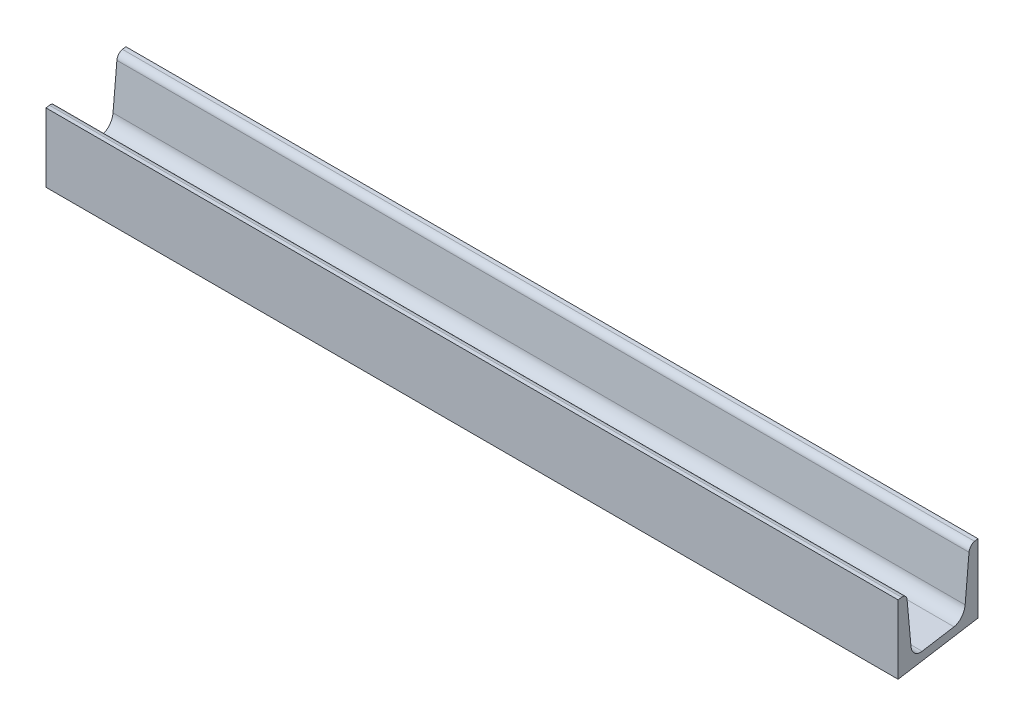
SolidWorks part; units mm, degrees
material "AISI 304"
ref_plane "Front Plane" through (0, 0, 0) normal (0, 0, 1) x (1, 0, 0)
ref_plane "Top Plane" through (0, 0, 0) normal (0, 1, 0) x (1, 0, 0)
ref_plane "Right Plane" through (0, 0, 0) normal (1, 0, 0) x (0, 0, -1)
other "Configuration Table"
sketch "草图1" plane through (0, 0, 0) normal (0, 0, 1) x (1, 0, 0)
  line L0 (-500, 0) -> (500, 0)
  point P4 (0, 0)
  dimension "D1" = 1000
other "GB/T 707-1988 hot-rolled channel 05(1)"
ref_plane "Plane1" through (-500, 0, 0) normal (1, 0, 0) x (0, 1, 0)
sketch "Sketch1" plane through (-500, 0, 0) normal (1, 0, 0) x (0, 1, 0)
  line L0 (37, 50) -> (0, 50)
  line L1 (37, 0) -> (0, 0)
  line L2 (0, 50) -> (0, 0)
  line L3 (-9.5694, 25) -> (49.7414, 25) construction
  line L4 (4.5, 34.9892) -> (4.5, 15.0108)
  line L5 (37, 0) -> (37, 2.1406)
  line L6 (37, 50) -> (37, 47.8594)
  line L7 (10.7683, 8.0491) -> (33.8658, 5.6215)
  line L17 (10.7683, 41.9509) -> (33.8658, 44.3785)
  arc A0 (33.8658, 44.3785) -> (37, 47.8594) centre (33.5, 47.8594) ccw
  arc A1 (33.8658, 5.6215) -> (37, 2.1406) centre (33.5, 2.1406) cw
  arc A2 (4.5, 15.0108) -> (10.7683, 8.0491) centre (11.5, 15.0108) ccw
  arc A10 (4.5, 34.9892) -> (10.7683, 41.9509) centre (11.5, 34.9892) cw
  point P6 (0, 0)
  point P8 (0, 25)
  point P9 (4.5, 25.8841)
  point P10 (18.5, 50)
  point P13 (37, 44.7079)
  point P14 (20.75, 43)
  point P19 (4.5, 25)
sketch "Sketch4" plane through (0, 0, 0) normal (0, -1, 0) x (1, 0, 0)
  line L0 (-500, 50) -> (-500, 0)
  line L1 (-500, 0) -> (-492.973, 50)
  line L2 (500, 50) -> (-500, 50) construction
  line L3 (-500, 50) -> (-492.973, 50)
  line L4 (500, 50) -> (-34.5112, 50)
  line L5 (-34.5112, 50) -> (-41.5383, 0)
  line L6 (-41.5383, 0) -> (500, 0)
  line L7 (500, 0) -> (500, 50)
  dimension "D1" = 8
  dimension "D2" = 454
extrude "Cut-Extrude6" cut sketch "Sketch4" against normal through all both and the other way through all
equation "\"RI@Sketch1\" = \"D1@Sketch1\""
equation "\"D3@Sketch1\" =  ( \"BF@Sketch1\" - \"D6@Sketch1\" )  / 2"
